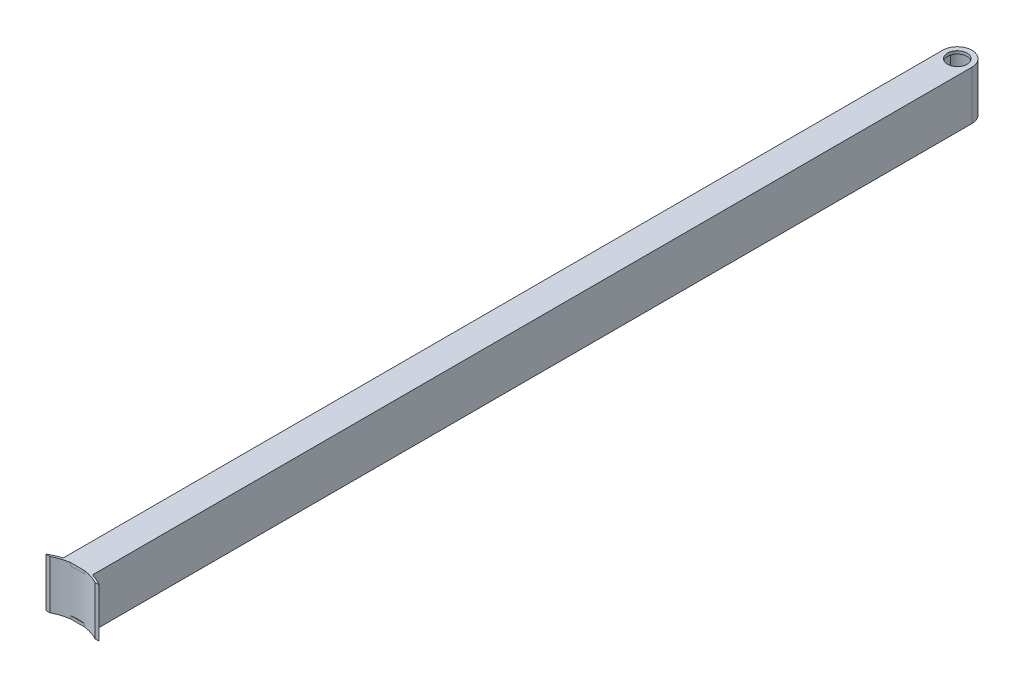
SolidWorks part; units mm, degrees
ref_plane "前视基准面" through (0, 0, 0) normal (0, 0, 1) x (1, 0, 0)
ref_plane "上视基准面" through (0, 0, 0) normal (0, 1, 0) x (1, 0, 0)
ref_plane "右视基准面" through (0, 0, 0) normal (1, 0, 0) x (0, 0, -1)
sketch "草图1" plane through (0, 0, 0) normal (0, 0, 1) x (1, 0, 0)
  line L0 (0, 0) -> (0, 50)
  line L1 (0, 50) -> (30, 50)
  line L2 (30, 50) -> (30, 0)
  line L3 (30, 0) -> (0, 0)
  line L4 (3, 3) -> (3, 47)
  line L5 (3, 47) -> (27, 47)
  line L6 (27, 47) -> (27, 3)
  line L7 (27, 3) -> (3, 3)
  dimension "D1" = 3
extrude "凸台-拉伸1" add sketch "草图1" along normal blind 900
sketch "草图2" plane through (0, 50, 0) normal (0, 1, 0) x (1, 0, 0)
  line L0 (15, 0) -> (15, -10)
  line L1 (30, 0) -> (0, 0) construction
  line L2 (15, 0) -> (15, -15)
  line L3 (0, -15) -> (0, 0)
  line L4 (0, 0) -> (30, 0)
  line L5 (30, -15) -> (30, 0)
  circle A0 centre (15, -15) radius 15
  circle A1 centre (15, -15) radius 10
extrude "切除-拉伸2" cut sketch "草图2" against normal blind 900
sketch "草图3" plane through (0, 50, 0) normal (0, 1, 0) x (1, 0, 0)
  line L0 (2, -15) -> (0, -15)
  line L1 (28, -15) -> (30, -15)
  arc A3 (28, -15) -> (2, -15) centre (15, -15) ccw
  arc A4 (28, -15) -> (2, -15) centre (15, -15) ccw
  arc A6 (30, -15) -> (0, -15) centre (15, -15) ccw
  arc A7 (30, -15) -> (0, -15) centre (15, -15) ccw
  dimension "D1" = 2
  dimension "D2" = 0
extrude "凸台-拉伸2" add sketch "草图3" against normal blind 50
sketch "草图4" plane through (0, 0, 900) normal (0, 0, 1) x (1, 0, 0)
  line L4 (3, 47) -> (3, 3)
  line L5 (3, 3) -> (27, 3)
  line L6 (27, 3) -> (27, 47)
  line L7 (27, 47) -> (3, 47)
  line L8 (0, 0) -> (30, 0)
  line L9 (30, 0) -> (30, 50)
  line L10 (30, 50) -> (0, 50)
  line L11 (0, 50) -> (0, 0)
  line L12 (0, 0) -> (30, 0)
  line L13 (30, 0) -> (30, 50)
  line L14 (30, 50) -> (0, 50)
  line L15 (0, 50) -> (0, 0)
  dimension "D1" = 0
extrude "凸台-拉伸3" add sketch "草图4" along normal blind 15
sketch "草图5" plane through (0, 50, 0) normal (0, 1, 0) x (1, 0, 0)
  line L2 (-12.2208, -920.0987) -> (-8.1287, -920.0987)
  line L3 (38.1287, -920.0987) -> (42.2208, -920.0987)
  arc A0 (42.2208, -920.0987) -> (-12.2208, -920.0987) centre (15, -965) ccw
  arc A4 (38.1287, -920.0987) -> (-8.1287, -920.0987) centre (15, -965) ccw
  arc A5 (41.1839, -921.8089) -> (-11.1839, -921.8089) centre (15, -965) ccw construction
  dimension "D2" = 2
extrude "凸台-拉伸4" add sketch "草图5" against normal blind 50
